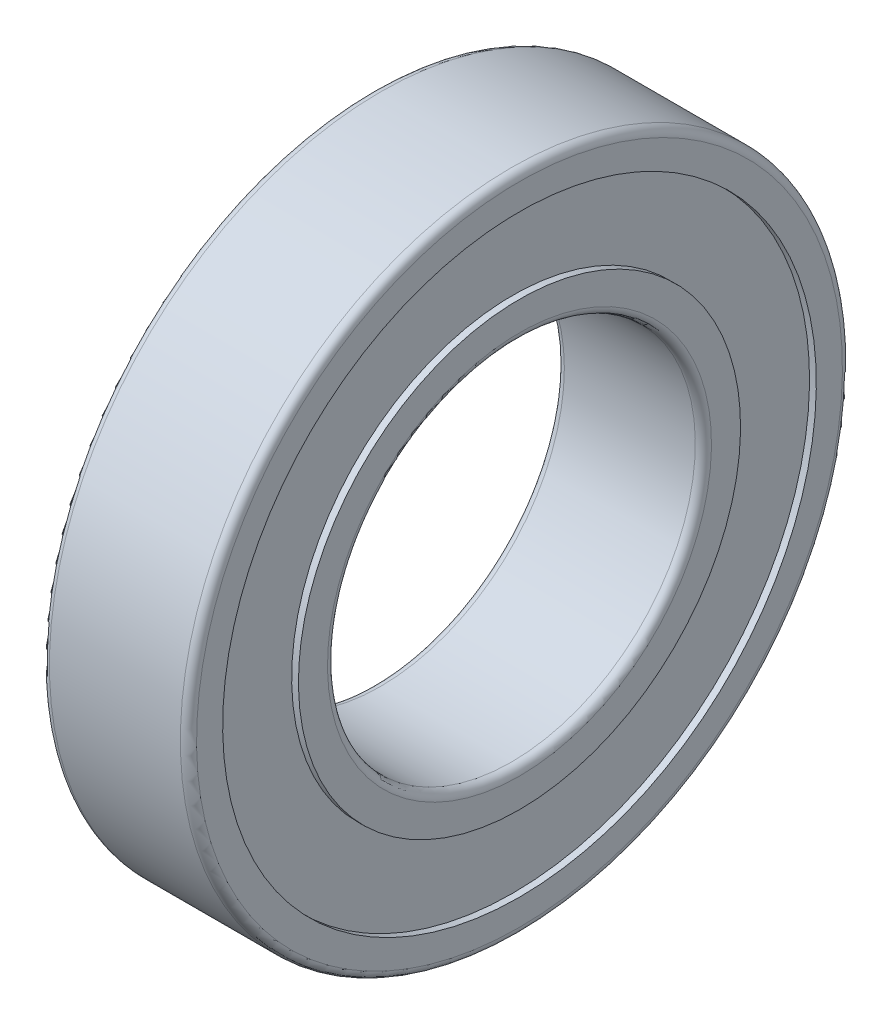
SolidWorks part; units mm, degrees
ref_plane "Front Plane" through (0, 0, 0) normal (0, 0, 1) x (1, 0, 0)
ref_plane "Top Plane" through (0, 0, 0) normal (0, 1, 0) x (1, 0, 0)
ref_plane "Right Plane" through (0, 0, 0) normal (1, 0, 0) x (0, 0, -1)
sketch "Sketch1" plane through (0, 0, 0) normal (0, 0, 1) x (1, 0, 0)
  line L0 (0, 0) -> (20, 0) construction
  line L1 (0, 25) -> (20, 25)
  line L2 (0, 45) -> (20, 45)
  line L3 (0, 45) -> (0, 40.35)
  line L4 (0, 40.35) -> (0.92, 40.35)
  line L5 (20, 45) -> (20, 40.35)
  line L6 (0.92, 40.35) -> (0.92, 30.05)
  line L7 (0.92, 30.05) -> (0, 30.05)
  line L8 (0, 30.05) -> (0, 25)
  line L9 (20, 40.35) -> (19.08, 40.35)
  line L10 (19.08, 40.35) -> (19.08, 30.05)
  line L11 (19.08, 30.05) -> (20, 30.05)
  line L12 (20, 30.05) -> (20, 25)
  dimension "D" = 90
  dimension "B" = 20
  dimension "D_s" = 50
  dimension "MSM_1" = 80.7
  dimension "MSM_2" = 60.1
  dimension "MSM_3" = 0.92
revolve "Revolve1" add sketch "Sketch1" angle 360 about L0
fillet "Fillet1" radius 1.1 2 edges at (20, -45, 0) (0, -45, 0)
fillet "Fillet2" radius 1.1 2 edges at (20, -25, 0) (0, -25, 0)
